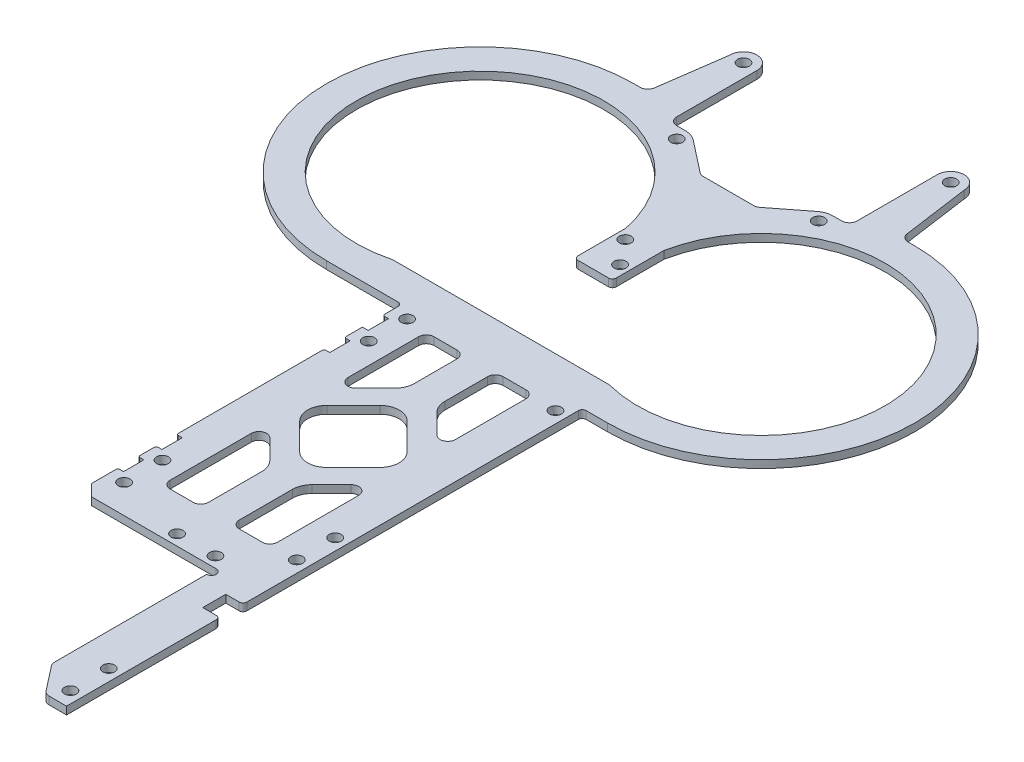
from build123d import *

# Parameters (mm, degrees)
SKETCH_1_R          = 1.55
EXTRUDE_1_DEPTH     = 2
SKETCH_3_R          = 1.25
SKETCH_3_W          = 1.5
SKETCH_3_H          = 5.3
SKETCH_3_W_2        = 4.5
SKETCH_3_H_2        = 6
CUT_EXTRUDE_1_DEPTH = 3.2
CHAMFER_1_SIZE      = 3
FILLET_1_R          = 2
FILLET_2_R          = 5
FILLET_3_R          = 0.5
FILLET_4_R          = 1


with BuildPart() as part:
    # 草图1 → 凸台-拉伸1 (new body)
    with BuildSketch(Plane(origin=(0, 0, 0), x_dir=(1, 0, 0), z_dir=(0, 1, 0))):
        with BuildLine():
            Line((17.5, 36.1), (23.5, 36.1))
            Line((23.5, 36.1), (23.5, 59))
            ThreePointArc((23.5, 59), (27, 62.5), (30.5, 59))
            Line((30.5, 59), (33.170275859, 40))
            Line((33.170275859, 40), (36.625, 40))
            ThreePointArc((36.625, 40), (76.625, 0), (36.625, -40))
            Line((36.625, -40), (30, -40))
            Line((30, -40), (30, -123.9))
            Line((30, -123.9), (30, -174.4))
            Line((30, -174.4), (24.5, -174.4))
            Line((24.5, -174.4), (18.5, -166.720350207))
            Line((18.5, -166.720350207), (18.5, -123.9))
            Line((18.5, -123.9), (-17, -123.9))
            Line((-17, -123.9), (-17, -40))
            Line((-17, -40), (-36.625, -40))
            ThreePointArc((-36.625, -40), (-76.625, 0), (-36.625, 40))
            Line((-36.625, 40), (-33.170275859, 40))
            Line((-33.170275859, 40), (-30.5, 59))
            ThreePointArc((-30.5, 59), (-27, 62.5), (-23.5, 59))
            Line((-23.5, 59), (-23.5, 36.1))
            Line((-23.5, 36.1), (-17.5, 36.1))
            Line((-17.5, 36.1), (-7.260466942, 28.1))
            Line((-7.260466942, 28.1), (7.260466942, 28.1))
            Line((7.260466942, 28.1), (17.5, 36.1))
        make_face()
        with Locations(Location((18.5, 33.1, 0), (0, 0, 270))):
            Circle(SKETCH_1_R, mode=Mode.SUBTRACT)
        with Locations(Location((-18.5, 33.1, 0), (0, 0, 90))):
            Circle(SKETCH_1_R, mode=Mode.SUBTRACT)
        with Locations(Location((27, -44, 0), (0, 0, 270))):
            Circle(SKETCH_1_R, mode=Mode.SUBTRACT)
        with Locations(Location((27, -101.4, 0), (0, 0, 270))):
            Circle(SKETCH_1_R, mode=Mode.SUBTRACT)
        with Locations(Location((27, -111.4, 0), (0, 0, 270))):
            Circle(SKETCH_1_R, mode=Mode.SUBTRACT)
        with Locations(Location((-13, -42.65, 0), (0, 0, 270))):
            Circle(SKETCH_1_R, mode=Mode.SUBTRACT)
        with Locations(Location((-13, -52.65, 0), (0, 0, 270))):
            Circle(SKETCH_1_R, mode=Mode.SUBTRACT)
        with Locations(Location((-13, -106.4, 0), (0, 0, 270))):
            Circle(SKETCH_1_R, mode=Mode.SUBTRACT)
        with Locations(Location((-13, -116.4, 0), (0, 0, 270))):
            Circle(SKETCH_1_R, mode=Mode.SUBTRACT)
        with Locations(Location((5.5, -121.1, 0), (0, 0, 270))):
            Circle(SKETCH_1_R, mode=Mode.SUBTRACT)
        with Locations(Location((15.5, -121.1, 0), (0, 0, 270))):
            Circle(SKETCH_1_R, mode=Mode.SUBTRACT)
        with Locations(Location((27, -160.4, 0), (0, 0, 270))):
            Circle(SKETCH_1_R, mode=Mode.SUBTRACT)
        with Locations(Location((27, -170.4, 0), (0, 0, 270))):
            Circle(SKETCH_1_R, mode=Mode.SUBTRACT)
        with Locations(Location((-2.5, 3.7, 0), (0, 0, 270))):
            Circle(SKETCH_1_R, mode=Mode.SUBTRACT)
        with Locations(Location((2.5, -2.65, 0), (0, 0, 270))):
            Circle(SKETCH_1_R, mode=Mode.SUBTRACT)
        with Locations(Location((-27, 59, 0), (0, 0, 270))):
            Circle(SKETCH_1_R, mode=Mode.SUBTRACT)
        with Locations(Location((27, 59, 0), (0, 0, 90))):
            Circle(SKETCH_1_R, mode=Mode.SUBTRACT)
        with BuildLine():
            Line((-5, 6.318375978), (-5, -7.15))
            Line((-5, -7.15), (5, -7.15))
            Line((5, -7.15), (5, 6.318375978))
            ThreePointArc((5, 6.318375978), (64.020088972, 17.016803466), (28.273952162, -31.15))
            Line((28.273952162, -31.15), (-28.273952162, -31.15))
            ThreePointArc((-28.273952162, -31.15), (-64.020088972, 17.016803466), (-5, 6.318375978))
        make_face(mode=Mode.SUBTRACT)
    extrude(amount=EXTRUDE_1_DEPTH)

    # 草图3 → 切除-拉伸1 (cut)
    with BuildSketch(Plane(origin=(0, 2, 0), x_dir=(1, 0, 0), z_dir=(0, 1, 0))):
        with Locations((18.5, -125.15)):
            Circle(SKETCH_3_R)
        with Locations((-16.25, -47.65)):
            Rectangle(SKETCH_3_W, SKETCH_3_H)
        with Locations((-16.25, -57.65)):
            Rectangle(SKETCH_3_W, SKETCH_3_H)
        with Locations((-16.25, -101.4)):
            Rectangle(SKETCH_3_W, SKETCH_3_H)
        with Locations((-16.25, -111.4)):
            Rectangle(SKETCH_3_W, SKETCH_3_H)
        with Locations((27.75, -131.4)):
            Rectangle(SKETCH_3_W_2, SKETCH_3_H_2)
        Polygon((6.5, -90.15), (20.5, -76.15), (6.5, -62.15), (-7.5, -76.15), align=None)
        Polygon((-7.5, -68.371825407), (2.5, -58.371825407), (2.5, -43.15), (-7.5, -43.15), align=None)
        Polygon((-7.5, -83.928174593), (-7.5, -111.9), (2.5, -111.9), (2.5, -93.928174593), align=None)
        Polygon((10.5, -93.928174593), (20.5, -83.928174593), (20.5, -111.9), (10.5, -111.9), align=None)
        Polygon((20.5, -43.15), (20.5, -68.371825407), (10.5, -58.371825407), (10.5, -43.15), align=None)
    extrude(amount=-CUT_EXTRUDE_1_DEPTH, mode=Mode.SUBTRACT)

    # 倒角1
    chamfer_1_edges = [part.edges().sort_by_distance(p)[0] for p in [
        (-17, 1, 123.9),
    ]]
    chamfer(chamfer_1_edges, length=CHAMFER_1_SIZE)

    # 圆角1
    fillet_1_edges = [part.edges().sort_by_distance(p)[0] for p in [
        (-7.5, 1, 43.15),
        (2.5, 1, 43.15),
        (-7.5, 1, 68.371825407),
        (2.5, 1, 111.9),
        (-7.5, 1, 111.9),
        (-7.5, 1, 83.928174593),
        (10.5, 1, 111.9),
        (20.5, 1, 83.928174593),
        (20.5, 1, 111.9),
        (10.5, 1, 43.15),
        (20.5, 1, 43.15),
        (20.5, 1, 68.371825407),
        (23.5, 1, -36.1),
        (33.170275859, 1, -40),
        (24.5, 1, 174.4),
        (18.5, 1, 166.720350207),
        (-33.170275859, 1, -40),
        (-23.5, 1, -36.1),
        (-7.260466942, 1, -28.1),
        (7.260466942, 1, -28.1),
        (-28.273952162, 1, 31.15),
        (28.273952162, 1, 31.15),
    ]]
    fillet(fillet_1_edges, radius=FILLET_1_R)

    # 圆角2
    fillet_2_edges = [part.edges().sort_by_distance(p)[0] for p in [
        (6.5, 1, 90.15),
        (-7.5, 1, 76.15),
        (6.5, 1, 62.15),
        (20.5, 1, 76.15),
        (2.5, 1, 58.371825407),
        (2.5, 1, 93.928174593),
        (10.5, 1, 93.928174593),
        (10.5, 1, 58.371825407),
        (17.5, 1, -36.1),
        (-17.5, 1, -36.1),
    ]]
    fillet(fillet_2_edges, radius=FILLET_2_R)

    # 圆角3
    fillet_3_edges = [part.edges().sort_by_distance(p)[0] for p in [
        (-17, 1, 45),
        (-17, 1, 60.3),
        (-17, 1, 55),
        (-17, 1, 104.05),
        (-17, 1, 98.75),
        (-17, 1, 114.05),
        (-17, 1, 108.75),
        (-16.25, 0, 50.3),
    ]]
    fillet(fillet_3_edges, radius=FILLET_3_R)

    # 圆角4
    fillet_4_edges = [part.edges().sort_by_distance(p)[0] for p in [
        (30, 1, 128.4),
        (30, 1, 134.4),
        (30, 1, 40),
        (-17, 1, 40),
        (-5, 1, -6.318375978),
        (5, 1, -6.318375978),
        (5, 1, 7.15),
        (-5, 1, 7.15),
    ]]
    fillet(fillet_4_edges, radius=FILLET_4_R)


solid = part.part
